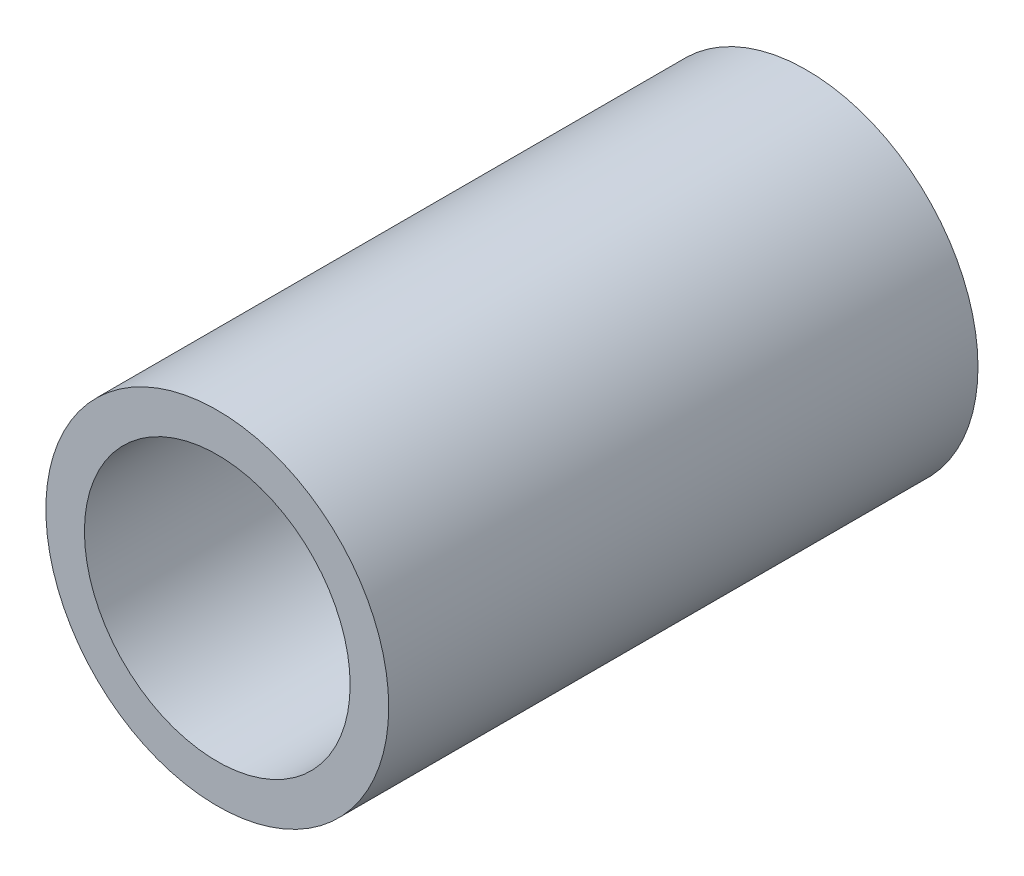
SolidWorks part; units mm, degrees
ref_plane "前视基准面" through (0, 0, 0) normal (0, 0, 1) x (1, 0, 0)
ref_plane "上视基准面" through (0, 0, 0) normal (0, 1, 0) x (1, 0, 0)
ref_plane "右视基准面" through (0, 0, 0) normal (1, 0, 0) x (0, 0, -1)
sketch "草图1" plane through (0, 0, 0) normal (0, 0, 1) x (1, 0, 0)
  circle A0 centre (0, 0) radius 12.4
  circle A1 centre (0, 0) radius 16
  dimension "外径" = 32
  dimension "壁厚" = 3.6
extrude "凸台-拉伸1" add sketch "草图1" along normal mid plane 55
